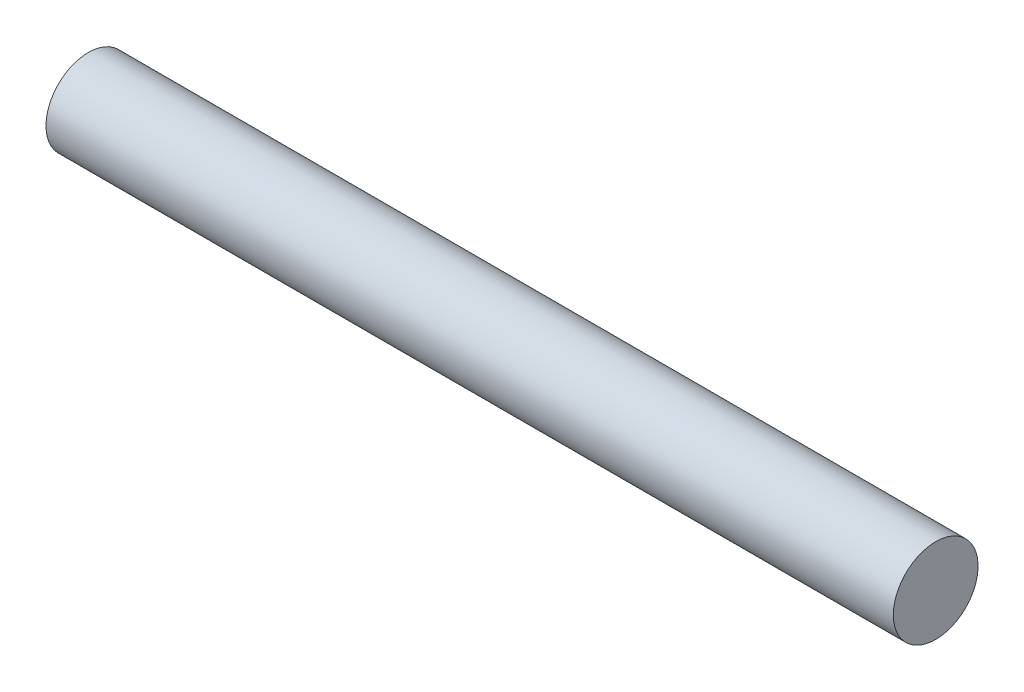
SolidWorks part; units mm, degrees
ref_plane "Front Plane" through (0, 0, 0) normal (0, 0, 1) x (1, 0, 0)
ref_plane "Top Plane" through (0, 0, 0) normal (0, 1, 0) x (1, 0, 0)
ref_plane "Right Plane" through (0, 0, 0) normal (1, 0, 0) x (0, 0, -1)
sketch "Sketch1" plane through (0, 0, 0) normal (0, 0, 1) x (1, 0, 0)
  line L0 (0, 0) -> (0, 1.5)
  line L1 (0, 0) -> (30, 0)
  line L3 (0, 1.5) -> (30, 1.5)
  line L4 (30, 0) -> (30, 1.5)
  dimension "D3" = 30
  dimension "D4" = 1.5
revolve "Revolve1" add sketch "Sketch1" angle 360 about L1
